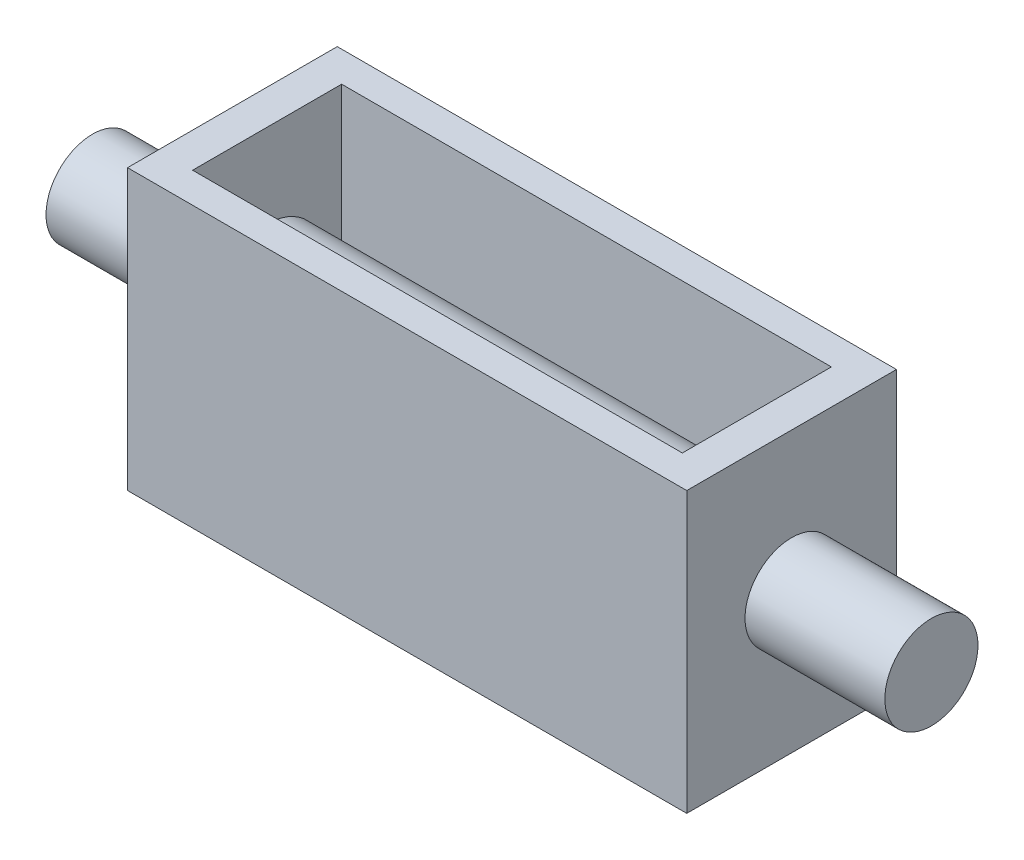
from build123d import *

# Parameters (mm, degrees)
SKETCH1_W           = 40
SKETCH1_H           = 15
BOSS_EXTRUDE1_DEPTH = 20
SKETCH2_W           = 35.032113562
SKETCH2_H           = 10.660333008
CUT_EXTRUDE1_DEPTH  = 10
SKETCH3_R           = 4
BOSS_EXTRUDE2_DEPTH = 35.032113562
SKETCH4_R           = 3.332307017
BOSS_EXTRUDE3_DEPTH = 10
BOSS_EXTRUDE4_START = 10
SKETCH5_R           = 3.332307017
BOSS_EXTRUDE4_DEPTH = 10
SCALE_1_SCALE       = 0.7


with BuildPart() as part:
    # Sketch1 → Boss-Extrude1 (new body)
    with BuildSketch(Plane(origin=(0, 0, 0), x_dir=(1, 0, 0), z_dir=(0, 1, 0))):
        Rectangle(SKETCH1_W, SKETCH1_H)
    extrude(amount=BOSS_EXTRUDE1_DEPTH)

    # Sketch2 → Cut-Extrude1 (cut)
    with BuildSketch(Plane(origin=(0, 20, 0), x_dir=(1, 0, 0), z_dir=(0, 1, 0))):
        Rectangle(SKETCH2_W, SKETCH2_H)
    extrude(amount=-CUT_EXTRUDE1_DEPTH, mode=Mode.SUBTRACT)

    # Sketch3 → Boss-Extrude2 (add)
    with BuildSketch(Plane(origin=(-17.516056781, 0, 0), x_dir=(0, 0, -1), z_dir=(1, 0, 0))):
        with Locations((0, 10)):
            Circle(SKETCH3_R)
    extrude(amount=BOSS_EXTRUDE2_DEPTH)

    # Sketch4 → Boss-Extrude3 (add)
    with BuildSketch(Plane.ZY.offset(20)):
        with Locations((0, 10)):
            Circle(SKETCH4_R)
    extrude(amount=BOSS_EXTRUDE3_DEPTH)

    # Sketch5 → Boss-Extrude4 (add)
    with BuildSketch(Plane(origin=(20, 0, 0), x_dir=(0, 0, -1), z_dir=(1, 0, 0)).offset(BOSS_EXTRUDE4_START)):
        with Locations(Location((0, 10, 0), (0, 0, 180))):
            Circle(SKETCH5_R)
    extrude(amount=-BOSS_EXTRUDE4_DEPTH)


with BuildPart() as part_1:
    # Scale 1: scaled about (0, 0, 0)
    add(part.part.scale(SCALE_1_SCALE))


solid = part_1.part
